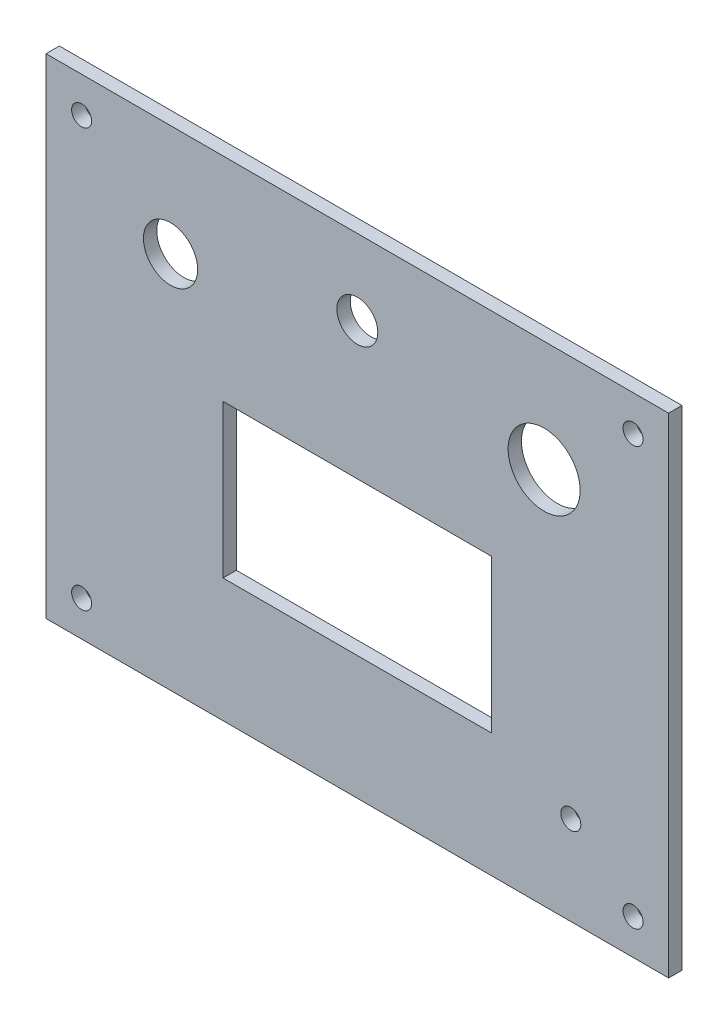
SolidWorks part; units mm, degrees
ref_plane "前视基准面" through (0, 0, 0) normal (0, 0, 1) x (1, 0, 0)
ref_plane "上视基准面" through (0, 0, 0) normal (0, 1, 0) x (1, 0, 0)
ref_plane "右视基准面" through (0, 0, 0) normal (1, 0, 0) x (0, 0, -1)
other "Configuration Table"
sketch "草图1" plane through (0, 0, 0) normal (0, 0, 1) x (1, 0, 0)
  line L0 (-70, -55) -> (70, -55)
  line L1 (70, -55) -> (70, 55)
  line L2 (70, 55) -> (-70, 55)
  line L3 (-70, 55) -> (-70, -55)
  line L4 (-30.2, -27.2) -> (30.2, -27.2)
  line L5 (30.2, -27.2) -> (30.2, 7.2)
  line L6 (30.2, 7.2) -> (-30.2, 7.2)
  line L7 (-30.2, 7.2) -> (-30.2, -27.2)
  circle A0 centre (-62, -47) radius 2.25
  circle A1 centre (-62, 47) radius 2.25
  circle A2 centre (62, -47) radius 2.25
  circle A3 centre (62, 47) radius 2.25
  circle A4 centre (-42, 30) radius 6.1
  circle A5 centre (42, 30) radius 8.1
  circle A6 centre (0, 38) radius 4.6
  circle A7 centre (48, -35) radius 2.25
  point P0 (0, 0)
  dimension "D1" = 12.2
  dimension "D2" = 4.5
  dimension "D3" = 4.5
  dimension "D4" = 16.2
  dimension "D5" = 4.5
  dimension "D6" = 4.5
  dimension "D7" = 9.2
  dimension "D8" = 4.5
  dimension "D9" = 8
  dimension "D10" = 22
  dimension "D11" = 28
  dimension "D12" = 39.8
  dimension "D13" = 70
  dimension "D14" = 100.2
  dimension "D15" = 112
  dimension "D16" = 132
  dimension "D17" = 140
  dimension "D18" = 8
  dimension "D19" = 17
  dimension "D20" = 25
  dimension "D21" = 47.8
  dimension "D22" = 55
  dimension "D23" = 82.2
  dimension "D24" = 90
  dimension "D25" = 102
  dimension "D26" = 110
extrude "凸台-拉伸1" add sketch "草图1" against normal mid plane 3
